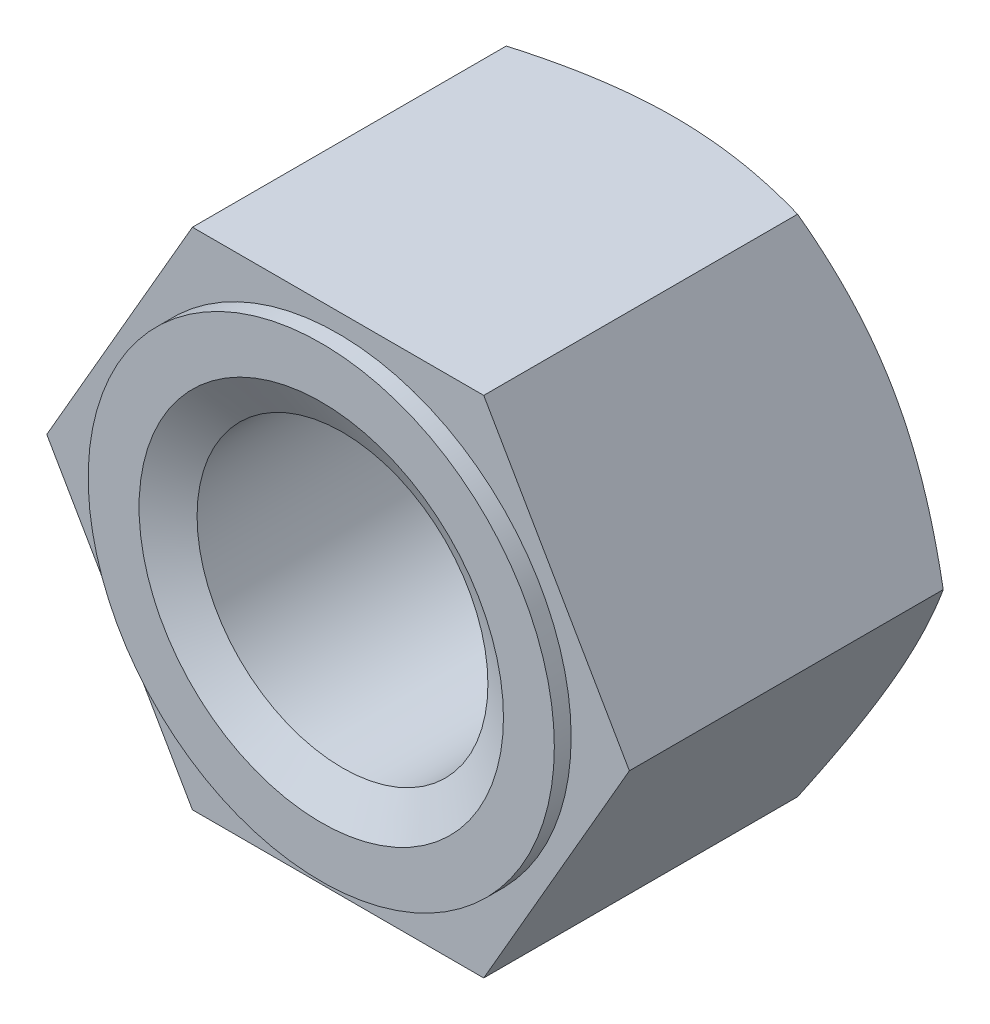
from build123d import *

# Parameters (mm, degrees)
SKETCH1_R         = 5.188
BASENUT_DEPTH     = 12
EXTRUDE1_START    = 0.6
SKETCH3_R         = 8.315
SKETCH3_R_2       = 5.188
EXTRUDE1_DEPTH    = 0.6
ENDCHAMFER3_SIZE  = 1.312
ENDCHAMFER3_SIZE2 = 0.757483553


with BuildPart() as part:
    # Sketch1 → BaseNut (new body)
    with BuildSketch(Plane.XY):
        Polygon((5.196152423, -9), (10.392304845, 0), (5.196152423, 9), (-5.196152423, 9), (-10.392304845, 0), (-5.196152423, -9), align=None)
        Circle(SKETCH1_R, mode=Mode.SUBTRACT)
    extrude(amount=-BASENUT_DEPTH)

    # Sketch2 → Chamfer1 (revolve, cut)
    with BuildSketch(Plane(origin=(-16.706149795, 0, -15.04811501), x_dir=(0, 0, 1), z_dir=(0, 1, 0))):
        Polygon((3.04811501, 25.706149795), (3.04811501, 27.098454641), (3.851962587, 27.098454641), align=None)
    revolve(axis=Axis((0, 0, -38.770766557), (0, 0, 1)), mode=Mode.SUBTRACT)

    # Sketch6 → EndChamfer1 (revolve, cut)
    with BuildSketch(Plane(origin=(-9.197458863, 0, -10.252541137), x_dir=(0, 0, 1), z_dir=(0, 1, 0))):
        Polygon((-1.747458863, 14.385458863), (-1.747458863, 15.697458863), (-0.989975309, 14.385458863), align=None)
    revolve(axis=Axis((0, 0, 13.104863586), (0, 0, -1)), mode=Mode.SUBTRACT)

    # Sketch3 → Extrude1 (add)
    with BuildSketch(Plane(origin=(-18.48918612, 11.17895969, 0), x_dir=(1, 0, 0), z_dir=(0, 0, 1)).offset(EXTRUDE1_START)):
        with Locations((18.48918612, -11.17895969)):
            Circle(SKETCH3_R)
        with Locations((18.48918612, -11.17895969)):
            Circle(SKETCH3_R_2, mode=Mode.SUBTRACT)
    extrude(amount=-EXTRUDE1_DEPTH)

    # EndChamfer3
    endchamfer3_edges = [part.edges().sort_by_distance(p)[0] for p in [
        (-5.188, 0, 0.6),
    ]]
    endchamfer3_side = [part.faces().sort_by_distance(p)[0] for p in [
        (-8.079816285, 0, 0.6),
    ]]
    chamfer(endchamfer3_edges, length=ENDCHAMFER3_SIZE, length2=ENDCHAMFER3_SIZE2, reference=endchamfer3_side[0])


solid = part.part
